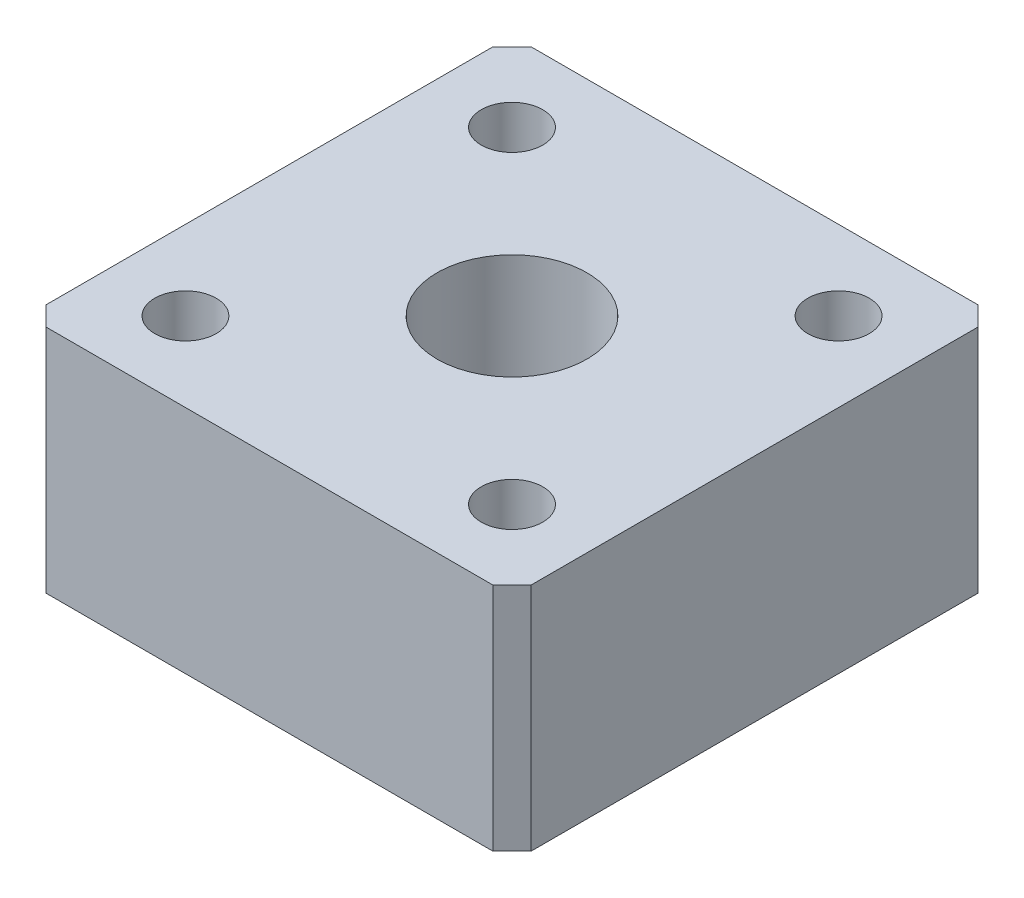
SolidWorks part; units mm, degrees
material "铜"
ref_plane "Front Plane" through (0, 0, 0) normal (0, 0, 1) x (1, 0, 0)
ref_plane "Top Plane" through (0, 0, 0) normal (0, 1, 0) x (1, 0, 0)
ref_plane "Right Plane" through (0, 0, 0) normal (1, 0, 0) x (0, 0, -1)
sketch "Sketch1" plane through (0, 0, 0) normal (0, 1, 0) x (1, 0, 0)
  line L0 (-6.315, 5.815) -> (-5.815, 6.315)
  line L1 (-5.815, -6.315) -> (5.815, -6.315)
  line L2 (-6.315, -5.815) -> (-6.315, 5.815)
  line L3 (-5.815, 6.315) -> (5.815, 6.315)
  line L4 (6.315, -5.815) -> (6.315, 5.815)
  line L5 (-6.315, -6.315) -> (6.315, 6.315) construction
  line L6 (-6.315, 6.315) -> (6.315, -6.315) construction
  line L7 (5.815, 6.315) -> (6.315, 5.815)
  line L8 (-6.315, -5.815) -> (-5.815, -6.315)
  line L9 (5.815, -6.315) -> (6.315, -5.815)
  circle A0 centre (0, 0) radius 1.95
  point P0 (0, 0)
  dimension "D2" = 3.9
  dimension "D1" = 12.63
extrude "Boss-Extrude1" add sketch "Sketch1" along normal blind 6
hole_wizard "M2 Tapped Hole2" positions "Sketch4" profile "Sketch3" tap size "M2" standard "GB"
sketch "Sketch4" plane through (0, 6, 0) normal (0, 1, 0) x (-1, 0, 0)
  point P209 (4.25, -4.25)
  point P212 (-4.25, -4.25)
  point P215 (-4.25, 4.25)
  point P218 (4.25, 4.25)
sketch "Sketch3" plane through (-4.25, 6, -4.25) normal (1, 0, 0) x (0, 0, 1)
  line L0 (0, 0) -> (0, 578.9574)
  line L1 (0, 578.9574) -> (0.8, 6)
  line L2 (0.8, 6) -> (0.8, 0)
  line L5 (0.8, 0) -> (0, 0)
  line L10 (0, 578.9574) -> (-0.8, 6) construction
  line L11 (0, -6.35) -> (0, 107.95) construction
  dimension "螺纹孔钻头直径" = 1.6
  dimension "螺纹孔钻头深度" = 6
  dimension "导头角度" = 0.16
cosmetic thread "CosmeticThread hole thread 1" parameters "D1"=4, "D2"=2
cosmetic thread "CosmeticThread hole thread 2" parameters "D1"=4, "D2"=2
cosmetic thread "CosmeticThread hole thread 3" parameters "D1"=4, "D2"=2
cosmetic thread "CosmeticThread hole thread 4" parameters "D1"=4, "D2"=2
